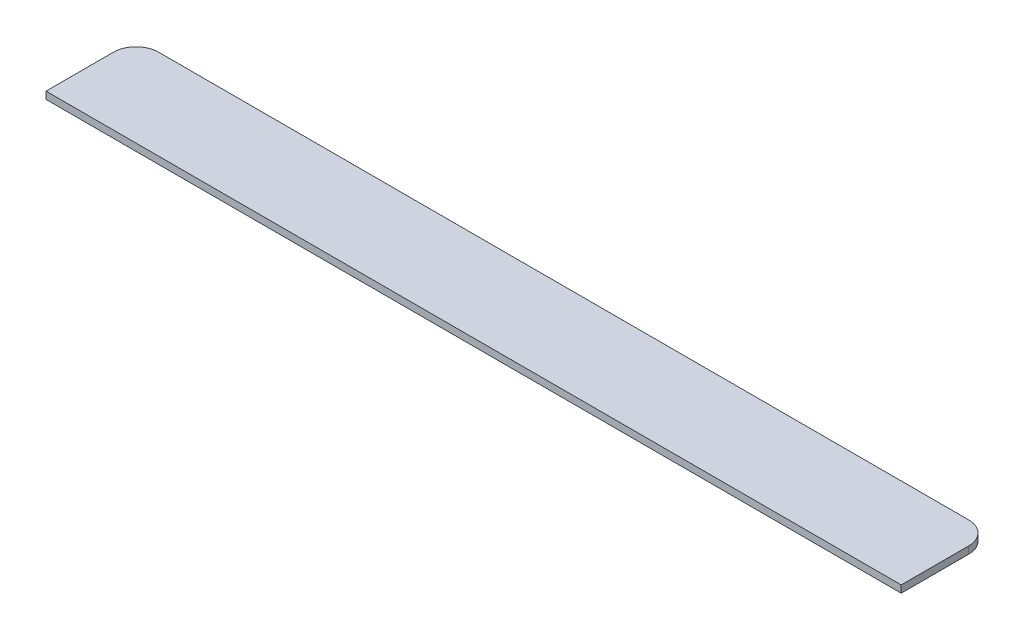
SolidWorks part; units mm, degrees
ref_plane "Front Plane" through (0, 0, 0) normal (0, 0, 1) x (1, 0, 0)
ref_plane "Top Plane" through (0, 0, 0) normal (0, 1, 0) x (1, 0, 0)
ref_plane "Right Plane" through (0, 0, 0) normal (1, 0, 0) x (0, 0, -1)
sketch "Sketch1" plane through (0, 0, 0) normal (0, 1, 0) x (1, 0, 0)
  line L1 (0, 0) -> (190, 0)
  line L2 (0, 0) -> (0, 15)
  line L3 (5, 20) -> (185, 20)
  line L4 (190, 0) -> (190, 15)
  arc A0 (185, 20) -> (190, 15) centre (185, 15) cw
  arc A1 (0, 15) -> (5, 20) centre (5, 15) cw
  point P9 (0, 20)
  dimension "D3" = 5
  dimension "D1" = 190
  dimension "D2" = 20
extrude "Boss-Extrude1" add sketch "Sketch1" along normal blind 1.6
